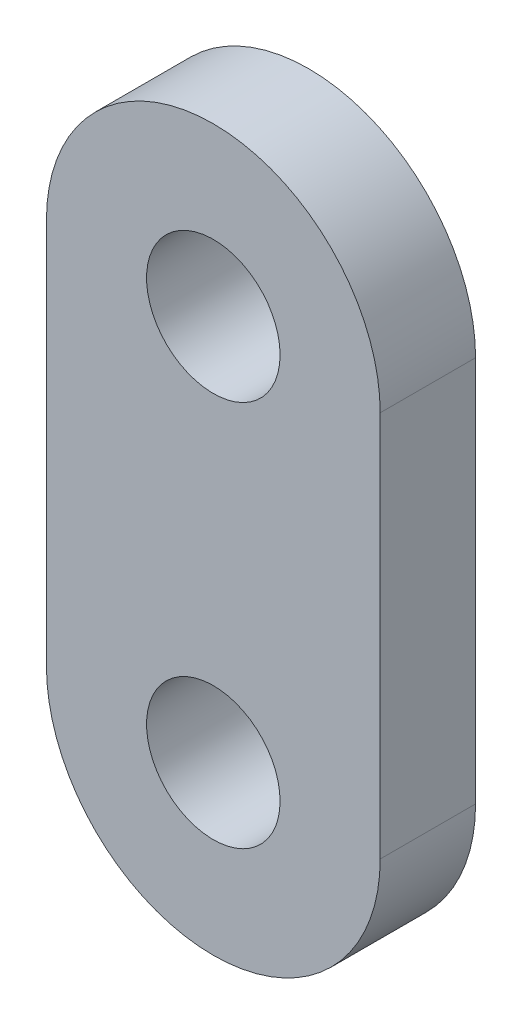
from build123d import *

# Parameters (mm, degrees)
SKETCH1_R           = 3.5
BOSS_EXTRUDE1_DEPTH = 5


with BuildPart() as part:
    # Sketch1 → Boss-Extrude1 (new body)
    with BuildSketch(Plane.XY):
        with BuildLine():
            Line((-8.75, 0), (-8.75, -20.26))
            ThreePointArc((-8.75, -20.26), (0, -29.01), (8.75, -20.26))
            Line((8.75, -20.26), (8.75, 0))
            ThreePointArc((8.75, 0), (0, 8.75), (-8.75, 0))
        make_face()
        Circle(SKETCH1_R, mode=Mode.SUBTRACT)
        with Locations((0, -20.26)):
            Circle(SKETCH1_R, mode=Mode.SUBTRACT)
    extrude(amount=BOSS_EXTRUDE1_DEPTH)


solid = part.part
